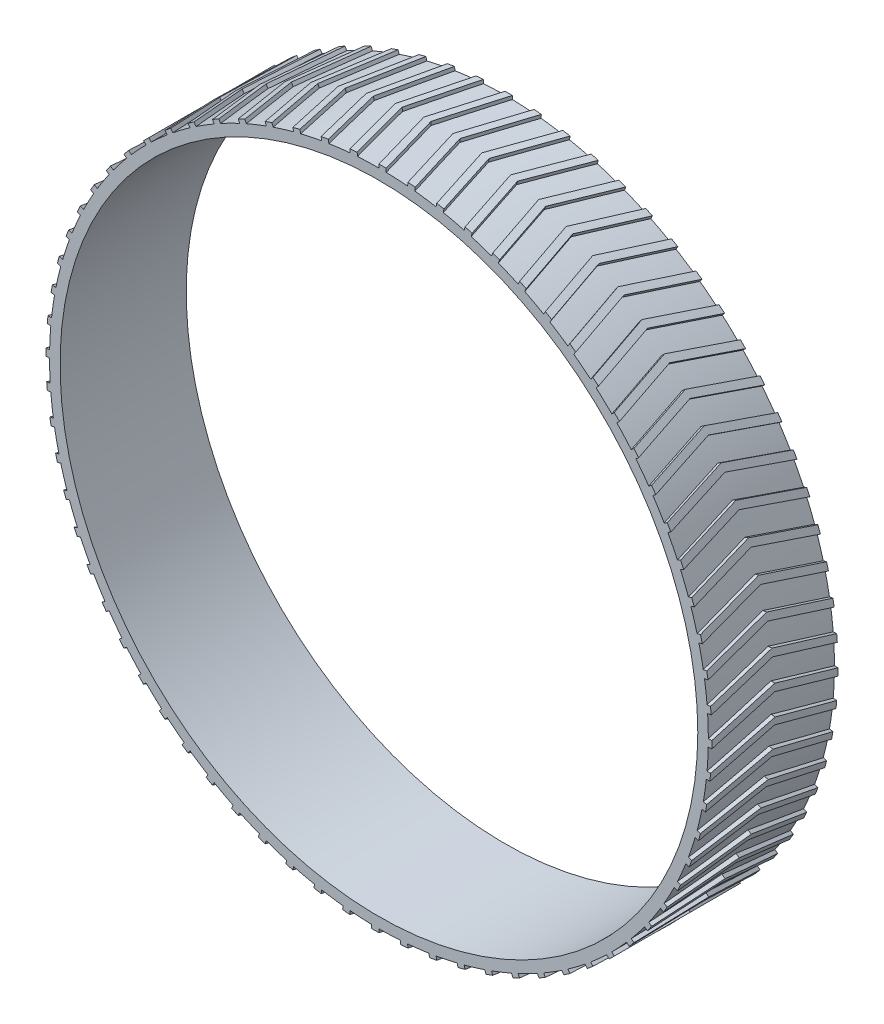
from build123d import *

# Parameters (mm, degrees)
SKETCH1_R           = 94
SKETCH1_R_2         = 91
BOSS_EXTRUDE1_DEPTH = 36
BOSS_EXTRUDE2_START = 92
BOSS_EXTRUDE2_DEPTH = 3
CIRPATTERN1_COUNT   = 72


with BuildPart() as part:
    # Sketch1 → Boss-Extrude1 (new body)
    with BuildSketch(Plane.XY):
        Circle(SKETCH1_R)
        Circle(SKETCH1_R_2, mode=Mode.SUBTRACT)
    extrude(amount=BOSS_EXTRUDE1_DEPTH)

    # Sketch3 → Boss-Extrude2 (add)
    with BuildSketch(Plane(origin=(0, 0, 0), x_dir=(1, 0, 0), z_dir=(0, 1, 0)).offset(BOSS_EXTRUDE2_START)):
        Polygon((0, 0), (-5.192850396, -18), (0, -36), (2.081564272, -36), (-3.111286124, -18), (2.081564272, 0), align=None)
    boss_extrude2 = extrude(amount=BOSS_EXTRUDE2_DEPTH)

    # CirPattern1: Boss-Extrude2 ×72 about axis
    cirpattern1_axis = Axis((0, 0, 0), (0, 0, 1))
    for i in range(1, CIRPATTERN1_COUNT):
        add(boss_extrude2.rotate(cirpattern1_axis, i * 360 / CIRPATTERN1_COUNT))


solid = part.part
